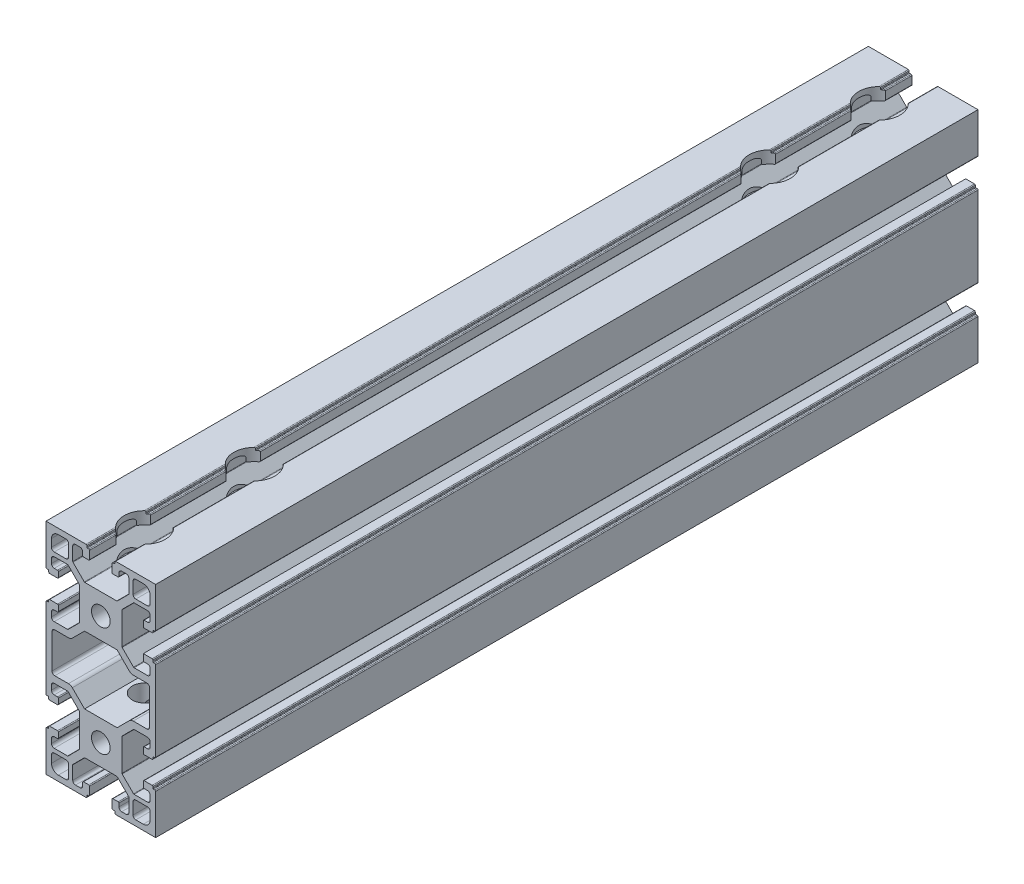
from build123d import *

# Parameters (mm, degrees)
MODEL_R                          = 3.4
EXTRUDE_1_DEPTH                  = 150
HOLE_WIZARD_2_D                  = 9
HOLE_WIZARD_2_CBORE_D            = 15
HOLE_WIZARD_2_CBORE_DEPTH        = 12.3
HOLE_WIZARD_M8_1_D               = 6.8
HOLE_WIZARD_M8_1_DEPTH           = 10.25
HOLE_WIZARD_M8_1_TIP             = 2.042926105
HOLE_WIZARD_M8_1_ON_FACE_2_D     = 6.8
HOLE_WIZARD_M8_1_ON_FACE_2_DEPTH = 10.25
HOLE_WIZARD_M8_1_ON_FACE_2_TIP   = 2.042926105


with BuildPart() as part:
    # Model → 凸台-拉伸1 (new, symmetric)
    with BuildSketch(Plane.XY):
        with BuildLine():
            Line((714.409918253, 268.229784956), (714.409918253, 266.329784956))
            ThreePointArc((714.409918253, 266.329784956), (714.322050287, 266.117652922), (714.109918253, 266.029784956))
            Line((714.109918253, 266.029784956), (711.209918253, 266.029784956))
            ThreePointArc((711.209918253, 266.029784956), (710.997786218, 266.117652922), (710.909918253, 266.329784956))
            Line((710.909918253, 266.329784956), (710.909918253, 266.829784956))
            ThreePointArc((710.909918253, 266.829784956), (710.851339609, 266.971206313), (710.709918253, 267.029784956))
            Line((710.709918253, 267.029784956), (710.209918253, 267.029784956))
            ThreePointArc((710.209918253, 267.029784956), (709.997786218, 267.117652922), (709.909918253, 267.329784956))
            Line((709.909918253, 267.329784956), (709.909918253, 281.929784956))
            Line((709.909918253, 281.929784956), (724.509918253, 281.929784956))
            ThreePointArc((724.509918253, 281.929784956), (724.722050287, 281.841916991), (724.809918253, 281.629784956))
            Line((724.809918253, 281.629784956), (724.809918253, 281.129784956))
            ThreePointArc((724.809918253, 281.129784956), (724.868496896, 280.9883636), (725.009918253, 280.929784956))
            Line((725.009918253, 280.929784956), (725.509918253, 280.929784956))
            ThreePointArc((725.509918253, 280.929784956), (725.722050287, 280.841916991), (725.809918253, 280.629784956))
            Line((725.809918253, 280.629784956), (725.809918253, 277.729784956))
            ThreePointArc((725.809918253, 277.729784956), (725.722050287, 277.517652922), (725.509918253, 277.429784956))
            Line((725.509918253, 277.429784956), (723.609918253, 277.429784956))
            ThreePointArc((723.609918253, 277.429784956), (723.397786218, 277.517652922), (723.309918253, 277.729784956))
            Line((723.309918253, 277.729784956), (723.309918253, 278.929784956))
            ThreePointArc((723.309918253, 278.929784956), (723.017025034, 279.636891738), (722.309918253, 279.929784956))
            Line((722.309918253, 279.929784956), (720.659918253, 279.929784956))
            ThreePointArc((720.659918253, 279.929784956), (719.952811471, 279.636891738), (719.659918253, 278.929784956))
            Line((719.659918253, 278.929784956), (719.659918253, 274.071815978))
            ThreePointArc((719.659918253, 274.071815978), (719.682754393, 273.957010948), (719.747786218, 273.859683944))
            Line((719.747786218, 273.859683944), (723.88981724, 269.717652922))
            ThreePointArc((723.88981724, 269.717652922), (723.987144245, 269.652621097), (724.101949274, 269.629784956))
            Line((724.101949274, 269.629784956), (735.717887231, 269.629784956))
            ThreePointArc((735.717887231, 269.629784956), (735.832692261, 269.652621097), (735.930019265, 269.717652922))
            Line((735.930019265, 269.717652922), (740.072050287, 273.859683944))
            ThreePointArc((740.072050287, 273.859683944), (740.137082112, 273.957010948), (740.159918253, 274.071815978))
            Line((740.159918253, 274.071815978), (740.159918253, 278.929784956))
            ThreePointArc((740.159918253, 278.929784956), (739.867025034, 279.636891738), (739.159918253, 279.929784956))
            Line((739.159918253, 279.929784956), (737.509918253, 279.929784956))
            ThreePointArc((737.509918253, 279.929784956), (736.802811471, 279.636891738), (736.509918253, 278.929784956))
            Line((736.509918253, 278.929784956), (736.509918253, 277.729784956))
            ThreePointArc((736.509918253, 277.729784956), (736.422050287, 277.517652922), (736.209918253, 277.429784956))
            Line((736.209918253, 277.429784956), (734.309918253, 277.429784956))
            ThreePointArc((734.309918253, 277.429784956), (734.097786218, 277.517652922), (734.009918253, 277.729784956))
            Line((734.009918253, 277.729784956), (734.009918253, 280.629784956))
            ThreePointArc((734.009918253, 280.629784956), (734.097786218, 280.841916991), (734.309918253, 280.929784956))
            Line((734.309918253, 280.929784956), (734.809918253, 280.929784956))
            ThreePointArc((734.809918253, 280.929784956), (734.951339609, 280.9883636), (735.009918253, 281.129784956))
            Line((735.009918253, 281.129784956), (735.009918253, 281.629784956))
            ThreePointArc((735.009918253, 281.629784956), (735.097786218, 281.841916991), (735.309918253, 281.929784956))
            Line((735.309918253, 281.929784956), (749.909918253, 281.929784956))
            Line((749.909918253, 281.929784956), (749.909918253, 267.329784956))
            ThreePointArc((749.909918253, 267.329784956), (749.822050287, 267.117652922), (749.609918253, 267.029784956))
            Line((749.609918253, 267.029784956), (749.109918253, 267.029784956))
            ThreePointArc((749.109918253, 267.029784956), (748.968496896, 266.971206313), (748.909918253, 266.829784956))
            Line((748.909918253, 266.829784956), (748.909918253, 266.329784956))
            ThreePointArc((748.909918253, 266.329784956), (748.822050287, 266.117652922), (748.609918253, 266.029784956))
            Line((748.609918253, 266.029784956), (745.709918253, 266.029784956))
            ThreePointArc((745.709918253, 266.029784956), (745.497786218, 266.117652922), (745.409918253, 266.329784956))
            Line((745.409918253, 266.329784956), (745.409918253, 268.229784956))
            ThreePointArc((745.409918253, 268.229784956), (745.497786218, 268.441916991), (745.709918253, 268.529784956))
            Line((745.709918253, 268.529784956), (746.909918253, 268.529784956))
            ThreePointArc((746.909918253, 268.529784956), (747.617025034, 268.822678175), (747.909918253, 269.529784956))
            Line((747.909918253, 269.529784956), (747.909918253, 271.179784956))
            ThreePointArc((747.909918253, 271.179784956), (747.617025034, 271.886891738), (746.909918253, 272.179784956))
            Line((746.909918253, 272.179784956), (742.051949274, 272.179784956))
            ThreePointArc((742.051949274, 272.179784956), (741.937144245, 272.156948816), (741.83981724, 272.091916991))
            Line((741.83981724, 272.091916991), (737.697786218, 267.949885969))
            ThreePointArc((737.697786218, 267.949885969), (737.632754393, 267.852558964), (737.609918253, 267.737753935))
            Line((737.609918253, 267.737753935), (737.609918253, 256.121815978))
            ThreePointArc((737.609918253, 256.121815978), (737.632754393, 256.007010948), (737.697786218, 255.909683944))
            Line((737.697786218, 255.909683944), (741.83981724, 251.767652922))
            ThreePointArc((741.83981724, 251.767652922), (741.937144245, 251.702621097), (742.051949274, 251.679784956))
            Line((742.051949274, 251.679784956), (746.909918253, 251.679784956))
            ThreePointArc((746.909918253, 251.679784956), (747.617025034, 251.972678175), (747.909918253, 252.679784956))
            Line((747.909918253, 252.679784956), (747.909918253, 254.329784956))
            ThreePointArc((747.909918253, 254.329784956), (747.617025034, 255.036891738), (746.909918253, 255.329784956))
            Line((746.909918253, 255.329784956), (745.409918253, 255.329784956))
            Line((745.409918253, 255.329784956), (745.409918253, 257.829784956))
            Line((745.409918253, 257.829784956), (748.609918253, 257.829784956))
            ThreePointArc((748.609918253, 257.829784956), (748.822050287, 257.741916991), (748.909918253, 257.529784956))
            Line((748.909918253, 257.529784956), (748.909918253, 257.029784956))
            ThreePointArc((748.909918253, 257.029784956), (748.968496896, 256.8883636), (749.109918253, 256.829784956))
            Line((749.109918253, 256.829784956), (749.609918253, 256.829784956))
            ThreePointArc((749.609918253, 256.829784956), (749.822050287, 256.741916991), (749.909918253, 256.529784956))
            Line((749.909918253, 256.529784956), (749.909918253, 241.929784956))
            Line((749.909918253, 241.929784956), (749.909918253, 227.329784956))
            ThreePointArc((749.909918253, 227.329784956), (749.822050287, 227.117652922), (749.609918253, 227.029784956))
            Line((749.609918253, 227.029784956), (749.109918253, 227.029784956))
            ThreePointArc((749.109918253, 227.029784956), (748.968496896, 226.971206313), (748.909918253, 226.829784956))
            Line((748.909918253, 226.829784956), (748.909918253, 226.329784956))
            ThreePointArc((748.909918253, 226.329784956), (748.822050287, 226.117652922), (748.609918253, 226.029784956))
            Line((748.609918253, 226.029784956), (745.709918253, 226.029784956))
            ThreePointArc((745.709918253, 226.029784956), (745.497786218, 226.117652922), (745.409918253, 226.329784956))
            Line((745.409918253, 226.329784956), (745.409918253, 228.229784956))
            ThreePointArc((745.409918253, 228.229784956), (745.497786218, 228.441916991), (745.709918253, 228.529784956))
            Line((745.709918253, 228.529784956), (746.909918253, 228.529784956))
            ThreePointArc((746.909918253, 228.529784956), (747.617025034, 228.822678175), (747.909918253, 229.529784956))
            Line((747.909918253, 229.529784956), (747.909918253, 231.179784956))
            ThreePointArc((747.909918253, 231.179784956), (747.617025034, 231.886891738), (746.909918253, 232.179784956))
            Line((746.909918253, 232.179784956), (742.051949274, 232.179784956))
            ThreePointArc((742.051949274, 232.179784956), (741.937144245, 232.156948816), (741.83981724, 232.091916991))
            Line((741.83981724, 232.091916991), (737.697786218, 227.949885969))
            ThreePointArc((737.697786218, 227.949885969), (737.632754393, 227.852558964), (737.609918253, 227.737753935))
            Line((737.609918253, 227.737753935), (737.609918253, 216.121815978))
            ThreePointArc((737.609918253, 216.121815978), (737.632754393, 216.007010948), (737.697786218, 215.909683944))
            Line((737.697786218, 215.909683944), (741.83981724, 211.767652922))
            ThreePointArc((741.83981724, 211.767652922), (741.937144245, 211.702621097), (742.051949274, 211.679784956))
            Line((742.051949274, 211.679784956), (746.909918253, 211.679784956))
            ThreePointArc((746.909918253, 211.679784956), (747.617025034, 211.972678175), (747.909918253, 212.679784956))
            Line((747.909918253, 212.679784956), (747.909918253, 214.329784956))
            ThreePointArc((747.909918253, 214.329784956), (747.617025034, 215.036891738), (746.909918253, 215.329784956))
            Line((746.909918253, 215.329784956), (745.709918253, 215.329784956))
            ThreePointArc((745.709918253, 215.329784956), (745.497786218, 215.417652922), (745.409918253, 215.629784956))
            Line((745.409918253, 215.629784956), (745.409918253, 217.529784956))
            ThreePointArc((745.409918253, 217.529784956), (745.497786218, 217.741916991), (745.709918253, 217.829784956))
            Line((745.709918253, 217.829784956), (748.609918253, 217.829784956))
            ThreePointArc((748.609918253, 217.829784956), (748.822050287, 217.741916991), (748.909918253, 217.529784956))
            Line((748.909918253, 217.529784956), (748.909918253, 217.029784956))
            ThreePointArc((748.909918253, 217.029784956), (748.968496896, 216.8883636), (749.109918253, 216.829784956))
            Line((749.109918253, 216.829784956), (749.609918253, 216.829784956))
            ThreePointArc((749.609918253, 216.829784956), (749.822050287, 216.741916991), (749.909918253, 216.529784956))
            Line((749.909918253, 216.529784956), (749.909918253, 201.929784956))
            Line((749.909918253, 201.929784956), (735.309918253, 201.929784956))
            ThreePointArc((735.309918253, 201.929784956), (735.097786218, 202.017652922), (735.009918253, 202.229784956))
            Line((735.009918253, 202.229784956), (735.009918253, 202.729784956))
            ThreePointArc((735.009918253, 202.729784956), (734.951339609, 202.871206313), (734.809918253, 202.929784956))
            Line((734.809918253, 202.929784956), (734.309918253, 202.929784956))
            ThreePointArc((734.309918253, 202.929784956), (734.097786218, 203.017652922), (734.009918253, 203.229784956))
            Line((734.009918253, 203.229784956), (734.009918253, 206.129784956))
            ThreePointArc((734.009918253, 206.129784956), (734.097786218, 206.341916991), (734.309918253, 206.429784956))
            Line((734.309918253, 206.429784956), (736.209918253, 206.429784956))
            ThreePointArc((736.209918253, 206.429784956), (736.422050287, 206.341916991), (736.509918253, 206.129784956))
            Line((736.509918253, 206.129784956), (736.509918253, 204.929784956))
            ThreePointArc((736.509918253, 204.929784956), (736.802811471, 204.222678175), (737.509918253, 203.929784956))
            Line((737.509918253, 203.929784956), (739.159918253, 203.929784956))
            ThreePointArc((739.159918253, 203.929784956), (739.867025034, 204.222678175), (740.159918253, 204.929784956))
            Line((740.159918253, 204.929784956), (740.159918253, 209.787753935))
            ThreePointArc((740.159918253, 209.787753935), (740.137082112, 209.902558964), (740.072050287, 209.999885969))
            Line((740.072050287, 209.999885969), (735.930019265, 214.141916991))
            ThreePointArc((735.930019265, 214.141916991), (735.832692261, 214.206948816), (735.717887231, 214.229784956))
            Line((735.717887231, 214.229784956), (724.101949274, 214.229784956))
            ThreePointArc((724.101949274, 214.229784956), (723.987144245, 214.206948816), (723.88981724, 214.141916991))
            Line((723.88981724, 214.141916991), (719.747786218, 209.999885969))
            ThreePointArc((719.747786218, 209.999885969), (719.682754393, 209.902558964), (719.659918253, 209.787753935))
            Line((719.659918253, 209.787753935), (719.659918253, 204.929784956))
            ThreePointArc((719.659918253, 204.929784956), (719.952811471, 204.222678175), (720.659918253, 203.929784956))
            Line((720.659918253, 203.929784956), (722.309918253, 203.929784956))
            ThreePointArc((722.309918253, 203.929784956), (723.017025034, 204.222678175), (723.309918253, 204.929784956))
            Line((723.309918253, 204.929784956), (723.309918253, 206.129784956))
            ThreePointArc((723.309918253, 206.129784956), (723.397786218, 206.341916991), (723.609918253, 206.429784956))
            Line((723.609918253, 206.429784956), (725.509918253, 206.429784956))
            ThreePointArc((725.509918253, 206.429784956), (725.722050287, 206.341916991), (725.809918253, 206.129784956))
            Line((725.809918253, 206.129784956), (725.809918253, 203.229784956))
            ThreePointArc((725.809918253, 203.229784956), (725.722050287, 203.017652922), (725.509918253, 202.929784956))
            Line((725.509918253, 202.929784956), (725.009918253, 202.929784956))
            ThreePointArc((725.009918253, 202.929784956), (724.868496896, 202.871206313), (724.809918253, 202.729784956))
            Line((724.809918253, 202.729784956), (724.809918253, 202.229784956))
            ThreePointArc((724.809918253, 202.229784956), (724.722050287, 202.017652922), (724.509918253, 201.929784956))
            Line((724.509918253, 201.929784956), (709.909918253, 201.929784956))
            Line((709.909918253, 201.929784956), (709.909918253, 216.529784956))
            ThreePointArc((709.909918253, 216.529784956), (709.997786218, 216.741916991), (710.209918253, 216.829784956))
            Line((710.209918253, 216.829784956), (710.709918253, 216.829784956))
            ThreePointArc((710.709918253, 216.829784956), (710.851339609, 216.8883636), (710.909918253, 217.029784956))
            Line((710.909918253, 217.029784956), (710.909918253, 217.529784956))
            ThreePointArc((710.909918253, 217.529784956), (710.997786218, 217.741916991), (711.209918253, 217.829784956))
            Line((711.209918253, 217.829784956), (714.109918253, 217.829784956))
            ThreePointArc((714.109918253, 217.829784956), (714.322050287, 217.741916991), (714.409918253, 217.529784956))
            Line((714.409918253, 217.529784956), (714.409918253, 215.629784956))
            ThreePointArc((714.409918253, 215.629784956), (714.322050287, 215.417652922), (714.109918253, 215.329784956))
            Line((714.109918253, 215.329784956), (712.909918253, 215.329784956))
            ThreePointArc((712.909918253, 215.329784956), (712.202811471, 215.036891738), (711.909918253, 214.329784956))
            Line((711.909918253, 214.329784956), (711.909918253, 212.679784956))
            ThreePointArc((711.909918253, 212.679784956), (712.202811471, 211.972678175), (712.909918253, 211.679784956))
            Line((712.909918253, 211.679784956), (717.767887231, 211.679784956))
            ThreePointArc((717.767887231, 211.679784956), (717.882692261, 211.702621097), (717.980019265, 211.767652922))
            Line((717.980019265, 211.767652922), (722.122050287, 215.909683944))
            ThreePointArc((722.122050287, 215.909683944), (722.187082112, 216.007010948), (722.209918253, 216.121815978))
            Line((722.209918253, 216.121815978), (722.209918253, 227.737753935))
            ThreePointArc((722.209918253, 227.737753935), (722.187082112, 227.852558964), (722.122050287, 227.949885969))
            Line((722.122050287, 227.949885969), (717.980019265, 232.091916991))
            ThreePointArc((717.980019265, 232.091916991), (717.882692261, 232.156948816), (717.767887231, 232.179784956))
            Line((717.767887231, 232.179784956), (712.909918253, 232.179784956))
            ThreePointArc((712.909918253, 232.179784956), (712.202811471, 231.886891738), (711.909918253, 231.179784956))
            Line((711.909918253, 231.179784956), (711.909918253, 229.529784956))
            ThreePointArc((711.909918253, 229.529784956), (712.202811471, 228.822678175), (712.909918253, 228.529784956))
            Line((712.909918253, 228.529784956), (714.109918253, 228.529784956))
            ThreePointArc((714.109918253, 228.529784956), (714.322050287, 228.441916991), (714.409918253, 228.229784956))
            Line((714.409918253, 228.229784956), (714.409918253, 226.329784956))
            ThreePointArc((714.409918253, 226.329784956), (714.322050287, 226.117652922), (714.109918253, 226.029784956))
            Line((714.109918253, 226.029784956), (711.209918253, 226.029784956))
            ThreePointArc((711.209918253, 226.029784956), (710.997786218, 226.117652922), (710.909918253, 226.329784956))
            Line((710.909918253, 226.329784956), (710.909918253, 226.829784956))
            ThreePointArc((710.909918253, 226.829784956), (710.851339609, 226.971206313), (710.709918253, 227.029784956))
            Line((710.709918253, 227.029784956), (710.209918253, 227.029784956))
            ThreePointArc((710.209918253, 227.029784956), (709.997786218, 227.117652922), (709.909918253, 227.329784956))
            Line((709.909918253, 227.329784956), (709.909918253, 241.929784956))
            Line((709.909918253, 241.929784956), (709.909918253, 256.529784956))
            ThreePointArc((709.909918253, 256.529784956), (709.997786218, 256.741916991), (710.209918253, 256.829784956))
            Line((710.209918253, 256.829784956), (710.709918253, 256.829784956))
            ThreePointArc((710.709918253, 256.829784956), (710.851339609, 256.8883636), (710.909918253, 257.029784956))
            Line((710.909918253, 257.029784956), (710.909918253, 257.529784956))
            ThreePointArc((710.909918253, 257.529784956), (710.997786218, 257.741916991), (711.209918253, 257.829784956))
            Line((711.209918253, 257.829784956), (714.109918253, 257.829784956))
            ThreePointArc((714.109918253, 257.829784956), (714.322050287, 257.741916991), (714.409918253, 257.529784956))
            Line((714.409918253, 257.529784956), (714.409918253, 255.629784956))
            ThreePointArc((714.409918253, 255.629784956), (714.322050287, 255.417652922), (714.109918253, 255.329784956))
            Line((714.109918253, 255.329784956), (712.909918253, 255.329784956))
            ThreePointArc((712.909918253, 255.329784956), (712.202811471, 255.036891738), (711.909918253, 254.329784956))
            Line((711.909918253, 254.329784956), (711.909918253, 252.679784956))
            ThreePointArc((711.909918253, 252.679784956), (712.202811471, 251.972678175), (712.909918253, 251.679784956))
            Line((712.909918253, 251.679784956), (717.767887231, 251.679784956))
            ThreePointArc((717.767887231, 251.679784956), (717.882692261, 251.702621097), (717.980019265, 251.767652922))
            Line((717.980019265, 251.767652922), (722.122050287, 255.909683944))
            ThreePointArc((722.122050287, 255.909683944), (722.187082112, 256.007010948), (722.209918253, 256.121815978))
            Line((722.209918253, 256.121815978), (722.209918253, 267.737753935))
            ThreePointArc((722.209918253, 267.737753935), (722.187082112, 267.852558964), (722.122050287, 267.949885969))
            Line((722.122050287, 267.949885969), (717.980019265, 272.091916991))
            ThreePointArc((717.980019265, 272.091916991), (717.882692261, 272.156948816), (717.767887231, 272.179784956))
            Line((717.767887231, 272.179784956), (712.909918253, 272.179784956))
            ThreePointArc((712.909918253, 272.179784956), (712.202811471, 271.886891738), (711.909918253, 271.179784956))
            Line((711.909918253, 271.179784956), (711.909918253, 269.529784956))
            ThreePointArc((711.909918253, 269.529784956), (712.202811471, 268.822678175), (712.909918253, 268.529784956))
            Line((712.909918253, 268.529784956), (714.109918253, 268.529784956))
            ThreePointArc((714.109918253, 268.529784956), (714.322050287, 268.441916991), (714.409918253, 268.229784956))
        make_face()
        with Locations((729.909918253, 261.929784956)):
            Circle(MODEL_R, mode=Mode.SUBTRACT)
        with Locations((729.909918253, 221.929784956)):
            Circle(MODEL_R, mode=Mode.SUBTRACT)
        with BuildLine():
            Line((718.099258081, 234.679784956), (713.109918253, 234.679784956))
            ThreePointArc((713.109918253, 234.679784956), (712.402811471, 234.972678175), (712.109918253, 235.679784956))
            Line((712.109918253, 235.679784956), (712.109918253, 241.929784956))
            Line((712.109918253, 241.929784956), (712.109918253, 248.179784956))
            ThreePointArc((712.109918253, 248.179784956), (712.402811471, 248.886891738), (713.109918253, 249.179784956))
            Line((713.109918253, 249.179784956), (718.099258081, 249.179784956))
            ThreePointArc((718.099258081, 249.179784956), (718.864624946, 249.332025891), (719.513471643, 249.765571394))
            Line((719.513471643, 249.765571394), (723.977685206, 254.229784956))
            Line((723.977685206, 254.229784956), (735.8421513, 254.229784956))
            Line((735.8421513, 254.229784956), (740.306364862, 249.765571394))
            ThreePointArc((740.306364862, 249.765571394), (740.95521156, 249.332025891), (741.720578424, 249.179784956))
            Line((741.720578424, 249.179784956), (746.709918253, 249.179784956))
            ThreePointArc((746.709918253, 249.179784956), (747.417025034, 248.886891738), (747.709918253, 248.179784956))
            Line((747.709918253, 248.179784956), (747.709918253, 241.929784956))
            Line((747.709918253, 241.929784956), (747.709918253, 235.679784956))
            ThreePointArc((747.709918253, 235.679784956), (747.417025034, 234.972678175), (746.709918253, 234.679784956))
            Line((746.709918253, 234.679784956), (741.720578424, 234.679784956))
            ThreePointArc((741.720578424, 234.679784956), (740.95521156, 234.527544021), (740.306364862, 234.093998519))
            Line((740.306364862, 234.093998519), (735.8421513, 229.629784956))
            Line((735.8421513, 229.629784956), (723.977685206, 229.629784956))
            Line((723.977685206, 229.629784956), (719.513471643, 234.093998519))
            ThreePointArc((719.513471643, 234.093998519), (718.864624946, 234.527544021), (718.099258081, 234.679784956))
        make_face(mode=Mode.SUBTRACT)
        with BuildLine():
            Line((718.159918253, 278.929784956), (718.159918253, 274.679784956))
            ThreePointArc((718.159918253, 274.679784956), (717.867025034, 273.972678175), (717.159918253, 273.679784956))
            Line((717.159918253, 273.679784956), (712.909918253, 273.679784956))
            ThreePointArc((712.909918253, 273.679784956), (712.202811471, 273.972678175), (711.909918253, 274.679784956))
            Line((711.909918253, 274.679784956), (711.909918253, 277.429784956))
            ThreePointArc((711.909918253, 277.429784956), (712.6421513, 279.197551909), (714.409918252, 279.929784956))
            Line((714.409918252, 279.929784956), (717.159918253, 279.929784956))
            ThreePointArc((717.159918253, 279.929784956), (717.867025034, 279.636891738), (718.159918253, 278.929784956))
        make_face(mode=Mode.SUBTRACT)
        with BuildLine():
            Line((741.659918253, 278.929784956), (741.659918253, 274.679784956))
            ThreePointArc((741.659918253, 274.679784956), (741.952811471, 273.972678175), (742.659918253, 273.679784956))
            Line((742.659918253, 273.679784956), (746.909918253, 273.679784956))
            ThreePointArc((746.909918253, 273.679784956), (747.617025034, 273.972678175), (747.909918253, 274.679784956))
            Line((747.909918253, 274.679784956), (747.909918253, 277.429784956))
            ThreePointArc((747.909918253, 277.429784956), (747.177685206, 279.197551909), (745.409918253, 279.929784956))
            Line((745.409918253, 279.929784956), (742.659918253, 279.929784956))
            ThreePointArc((742.659918253, 279.929784956), (741.952811471, 279.636891738), (741.659918253, 278.929784956))
        make_face(mode=Mode.SUBTRACT)
        with BuildLine():
            Line((711.909918253, 206.429784956), (711.909918253, 209.179784956))
            ThreePointArc((711.909918253, 209.179784956), (712.202811471, 209.886891738), (712.909918253, 210.179784956))
            Line((712.909918253, 210.179784956), (717.159918253, 210.179784956))
            ThreePointArc((717.159918253, 210.179784956), (717.867025034, 209.886891738), (718.159918253, 209.179784956))
            Line((718.159918253, 209.179784956), (718.159918253, 204.929784956))
            ThreePointArc((718.159918253, 204.929784956), (717.867025034, 204.222678175), (717.159918253, 203.929784956))
            Line((717.159918253, 203.929784956), (714.409918252, 203.929784956))
            ThreePointArc((714.409918252, 203.929784956), (712.6421513, 204.662018003), (711.909918253, 206.429784956))
        make_face(mode=Mode.SUBTRACT)
        with BuildLine():
            Line((742.659918253, 203.929784956), (745.409918253, 203.929784956))
            ThreePointArc((745.409918253, 203.929784956), (747.177685206, 204.662018003), (747.909918253, 206.429784956))
            Line((747.909918253, 206.429784956), (747.909918253, 209.179784956))
            ThreePointArc((747.909918253, 209.179784956), (747.617025034, 209.886891738), (746.909918253, 210.179784956))
            Line((746.909918253, 210.179784956), (742.659918253, 210.179784956))
            ThreePointArc((742.659918253, 210.179784956), (741.952811471, 209.886891738), (741.659918253, 209.179784956))
            Line((741.659918253, 209.179784956), (741.659918253, 204.929784956))
            ThreePointArc((741.659918253, 204.929784956), (741.952811471, 204.222678175), (742.659918253, 203.929784956))
        make_face(mode=Mode.SUBTRACT)
    extrude(amount=EXTRUDE_1_DEPTH, both=True)

    # 打孔尺寸(%根据)内六角圆柱头螺钉的类型2 (through all)
    with Locations(Plane(origin=(729.909918253, 281.929784956, -134), x_dir=(0, 0, 1), z_dir=(0, 1, 0))):
        with Locations((0, 0), (40, 0), (228, 0), (268, 0)):
            CounterBoreHole(HOLE_WIZARD_2_D / 2, HOLE_WIZARD_2_CBORE_D / 2, HOLE_WIZARD_2_CBORE_DEPTH)

    # M8 螺纹孔1
    with Locations(Plane(origin=(729.909918253, 261.929784956, 150), x_dir=(1, 0, 0), z_dir=(0, 0, 1))):
        with Locations((0, 0), (0, -40)):
            Hole(HOLE_WIZARD_M8_1_D / 2, depth=HOLE_WIZARD_M8_1_DEPTH)
            with Locations((0, 0, -(HOLE_WIZARD_M8_1_DEPTH + HOLE_WIZARD_M8_1_TIP / 2))):  # 118° drill point
                Cone(0, HOLE_WIZARD_M8_1_D / 2, HOLE_WIZARD_M8_1_TIP, mode=Mode.SUBTRACT)

    # M8 螺纹孔1 on face 2
    with Locations(Plane(origin=(729.909918253, 261.929784956, -150), x_dir=(1, 0, 0), z_dir=(0, 0, 1))):
        with Locations((0, 0), (0, -40)):
            Hole(HOLE_WIZARD_M8_1_ON_FACE_2_D / 2, depth=HOLE_WIZARD_M8_1_ON_FACE_2_DEPTH)
            with Locations((0, 0, -(HOLE_WIZARD_M8_1_ON_FACE_2_DEPTH + HOLE_WIZARD_M8_1_ON_FACE_2_TIP / 2))):  # 118° drill point
                Cone(0, HOLE_WIZARD_M8_1_ON_FACE_2_D / 2, HOLE_WIZARD_M8_1_ON_FACE_2_TIP, mode=Mode.SUBTRACT)


solid = part.part
